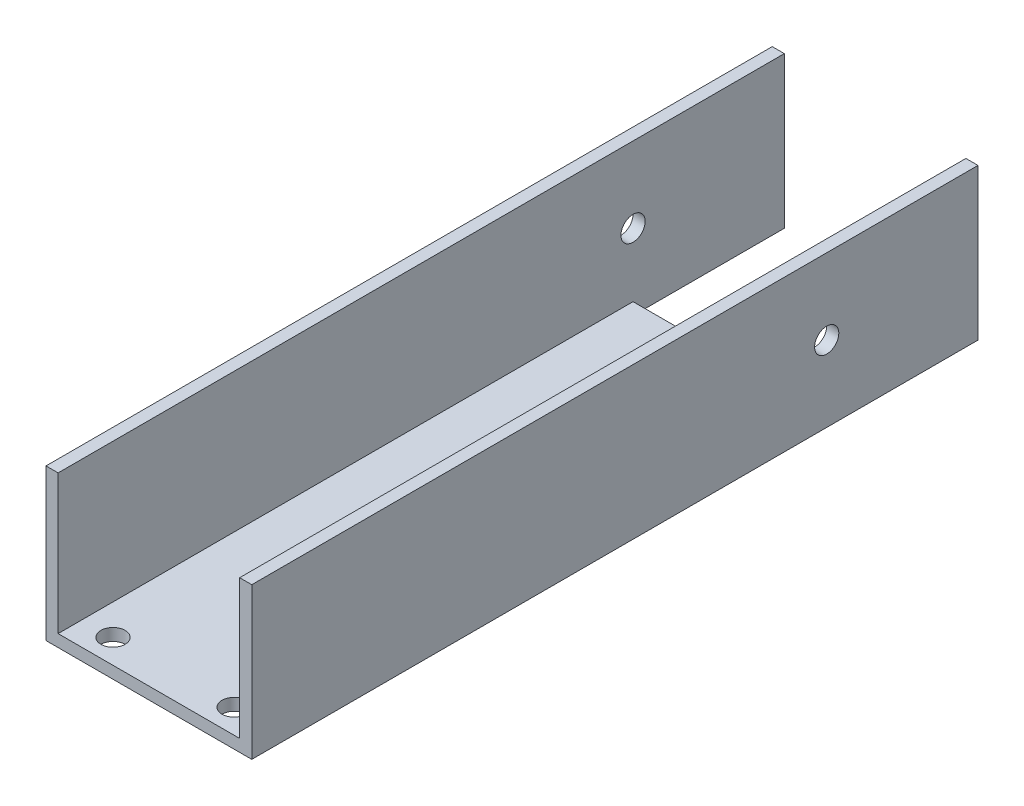
from build123d import *

# Parameters (mm, degrees)
BOSS_EXTRUDE1_DEPTH = 120
SKETCH2_R           = 2
CUT_EXTRUDE1_DEPTH  = 124.749747474
SKETCH3_W           = 30
SKETCH3_H           = 25
CUT_EXTRUDE2_DEPTH  = 124.3612581
SKETCH4_R           = 2
CUT_EXTRUDE3_DEPTH  = 127.82665335


with BuildPart() as part:
    # Sketch1 → Boss-Extrude1 (new body)
    with BuildSketch(Plane.XY):
        Polygon((-15, 23), (-15, 0), (15, 0), (15, 23), (17, 23), (17, -2), (-17, -2), (-17, 23), align=None)
    extrude(amount=BOSS_EXTRUDE1_DEPTH)

    # Sketch2 → Cut-Extrude1 (cut, through all)
    with BuildSketch(Plane.XZ.offset(2)):
        with Locations((0.071255778, 98.679491924)):
            Circle(SKETCH2_R)
        with Locations((10.071255778, 116)):
            Circle(SKETCH2_R)
        with Locations((-9.928744222, 116)):
            Circle(SKETCH2_R)
    extrude(amount=-CUT_EXTRUDE1_DEPTH, mode=Mode.SUBTRACT)

    # Sketch3 → Cut-Extrude2 (cut, through all)
    with BuildSketch(Plane(origin=(0, 0, 0), x_dir=(1, 0, 0), z_dir=(0, 1, 0))):
        with Locations((0, -12.5)):
            Rectangle(SKETCH3_W, SKETCH3_H)
    extrude(amount=-CUT_EXTRUDE2_DEPTH, mode=Mode.SUBTRACT)

    # Sketch4 → Cut-Extrude3 (cut, through all)
    with BuildSketch(Plane(origin=(17, 0, 0), x_dir=(0, 0, -1), z_dir=(1, 0, 0))):
        with Locations(Location((-25, 10.5, 0), (0, 0, 90))):
            Circle(SKETCH4_R)
    extrude(amount=-CUT_EXTRUDE3_DEPTH, mode=Mode.SUBTRACT)


solid = part.part
